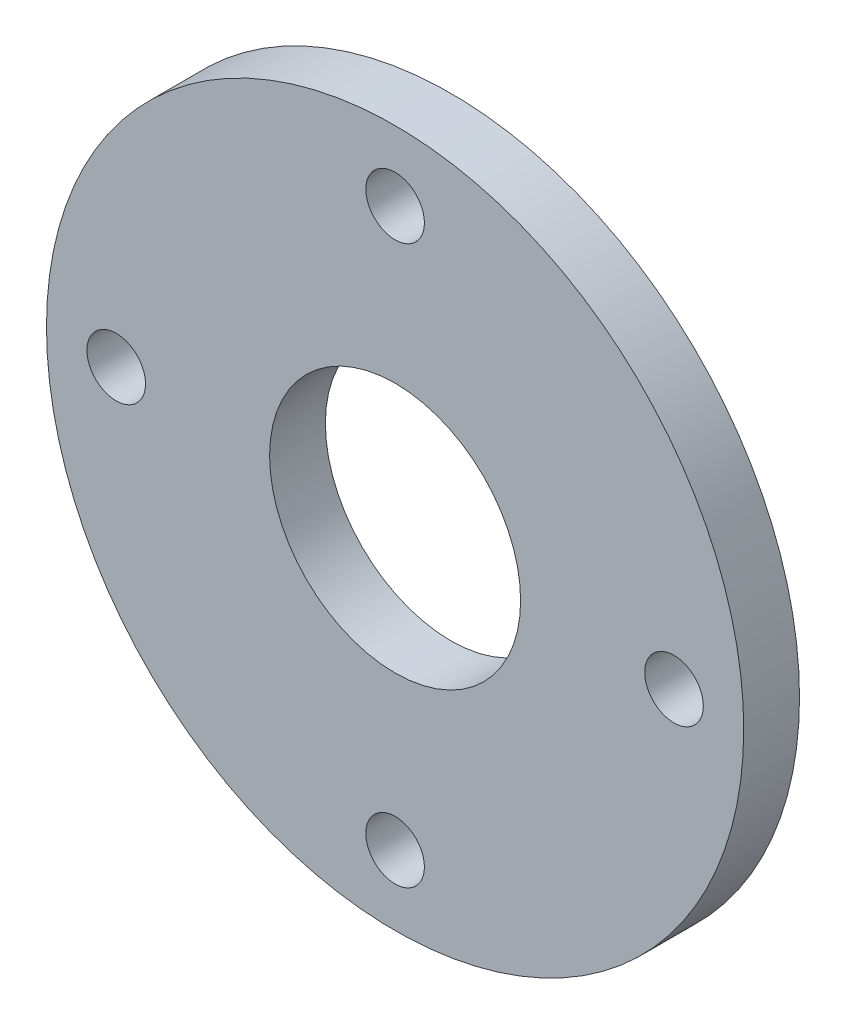
SolidWorks part; units mm, degrees
material "国产6061 "
ref_plane "Front Plane" through (0, 0, 0) normal (0, 0, 1) x (1, 0, 0)
ref_plane "Top Plane" through (0, 0, 0) normal (0, 1, 0) x (1, 0, 0)
ref_plane "Right Plane" through (0, 0, 0) normal (1, 0, 0) x (0, 0, -1)
sketch "Sketch1" plane through (0, 0, 0) normal (0, 0, 1) x (1, 0, 0)
  circle A0 centre (0, 0) radius 9
  circle A1 centre (0, 0) radius 25
  circle A2 centre (0, 0) radius 20 construction
  circle A3 centre (0, 20) radius 2.1
  circle A4 centre (-20, 0) radius 2.1
  circle A5 centre (20, 0) radius 2.1
  circle A6 centre (0, -20) radius 2.1
  dimension "D1" = 50
  dimension "D2" = 18
  dimension "D3" = 40
  dimension "D4" = 4.2
extrude "Boss-Extrude1" add sketch "Sketch1" along normal blind 4
